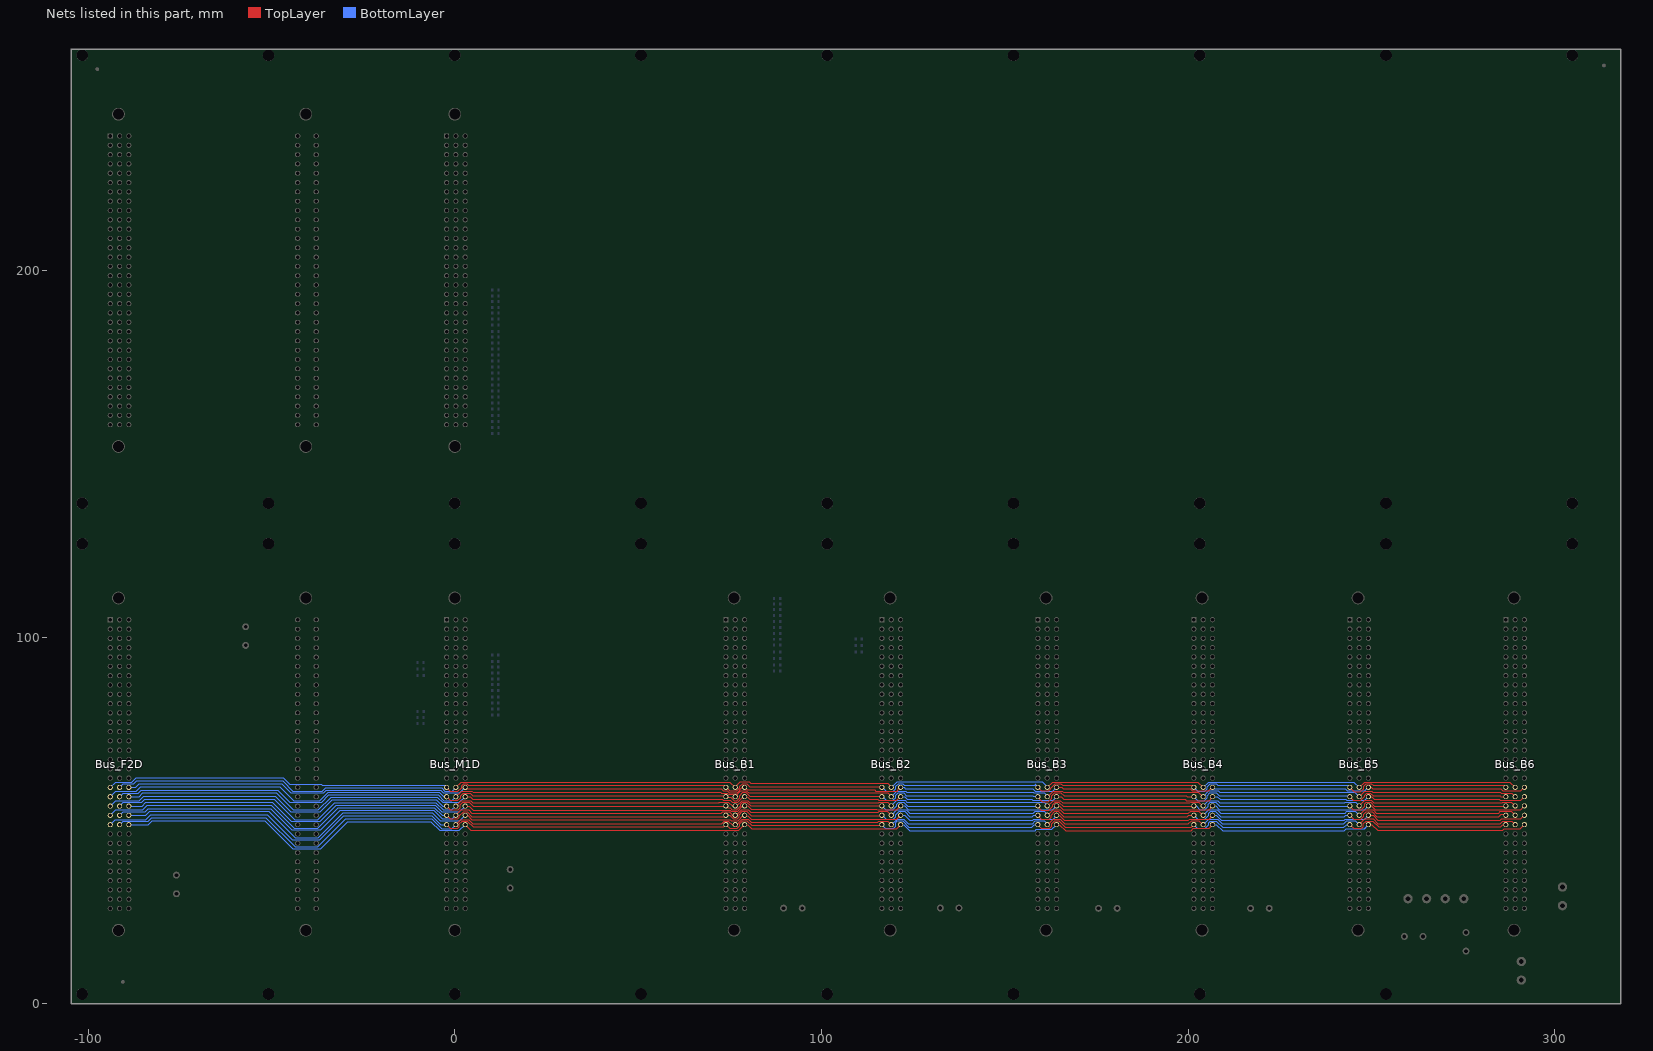
[diagram p0: the nets of this part, all layers, seen from the top]
# Altium PCB MISC67337.PcbDoc (part 3 of 7)
Units mm, origin at the board's own origin, x right, y up, seen from the top; angles counter-clockwise.
Board outline 422.71 x 260.35 mm, 4 copper layers (TopLayer, InternalPlane1, InternalPlane2, BottomLayer); 82 components, 143 nets, 1295 pads, 42 vias.

## Via types
v1: diameter 0.61, hole 0.305, TopLayer to BottomLayer, 42 vias

## Nets (pads, with @x,y where several pads share a name; then routed paths per layer and width w, separated by ;. In a path a pad name is that pad's centre, name@x,y a point inside that pad or via, vN(x,y) a via of type N, cw(c..) or ccw(c..) an arc to the next point about the centre after c; other vN are vias at no path point) (continued)
B_DSP1_XD0: Bus_B1.A19 Bus_B2.A19 Bus_B3.A19 Bus_B4.A19 Bus_B5.A19 Bus_B6.A19 Bus_F2D.A19 Bus_M1D.A19 | length 403.1
  TopLayer w0.254: Bus_M1D.A19@-2.24,58.974 -1.178,57.912 0.838,57.912 1.862,58.936 1.862,59.379 2.435,59.952 3.245,59.952 3.689,59.508 70.968,59.508 ; 72.996,59.508 70.968,59.508 ; Bus_B1.A19@73.955,58.993 73.44,59.508 70.968,59.508 ; Bus_B1.A19@73.96,59.12 75.065,58.015 76.9,58.015 77.785,58.9 77.785,59.248 78.508,59.971 79.704,59.971 80.457,59.217 Bus_B2.A19@116.505,59.217 ; Bus_B3.A19@159.05,58.993 160.004,58.039 161.036,58.039 161.06,58.015 161.995,58.015 162.568,58.588 162.568,58.814 163.774,60.02 165.329,60.02 165.849,59.499 168.021,59.499 ; 166.559,59.499 168.021,59.499 ; Bus_B4.A19@201.595,58.993 201.089,59.499 168.021,59.499 ; Bus_B5.A19@244.14,58.993 245.348,57.785 247.015,57.785 247.904,58.674 247.904,59.309 248.566,59.971 250.032,59.971 250.495,59.508 283.235,59.508 ; 283.945,59.508 283.235,59.508 ; Bus_B6.A19@286.685,58.993 286.17,59.508 283.235,59.508
  BottomLayer w0.254: Bus_F2D.A19@-93.97,58.974 -92.492,60.452 -88.138,60.452 -86.919,61.671 -46.838,61.671 -45.055,59.888 -36.47,59.888 -36.195,59.614 -2.88,59.614 Bus_M1D.A19@-2.24,58.974 ; Bus_B2.A19@116.632,59.055 117.713,57.974 119.634,57.974 120.269,58.609 120.269,59.244 121.058,60.033 122.162,60.033 122.631,59.564 155.981,59.564 ; 158.199,59.564 155.981,59.564 ; 158.199,60.033 Bus_B3.A19@159.177,59.055 ; Bus_B3.A19@159.05,58.993 158.479,59.564 155.981,59.564 ; Bus_B4.A19@201.595,58.993 202.676,57.912 204.597,57.912 205.232,58.547 205.232,59.182 206.021,59.971 207.635,59.971 208.102,59.504 242.519,59.504 ; 243.162,59.504 242.519,59.504 ; Bus_B5.A19@244.14,58.993 243.629,59.504 242.519,59.504
B_DSP1_XD1: Bus_B1.B19 Bus_B2.B19 Bus_B3.B19 Bus_B4.B19 Bus_B5.B19 Bus_B6.B19 Bus_F2D.B19 Bus_M1D.B19 | length 390.9
  TopLayer w0.254: Bus_M1D.B19@0.3,58.974 1.778,60.452 75.036,60.452 Bus_B1.B19@76.495,58.993 ; Bus_B1.B19@76.5,59.12 77.934,60.554 80.316,60.554 80.772,60.098 118.067,60.098 Bus_B2.B19@119.045,59.12 ; Bus_B3.B19@161.59,58.993 163.049,60.452 202.676,60.452 Bus_B4.B19@204.135,58.993 ; Bus_B5.B19@246.68,58.993 248.139,60.452 287.766,60.452 Bus_B6.B19@289.225,58.993
  BottomLayer w0.254: Bus_F2D.B19@-91.43,58.974 -90.452,59.952 -87.495,59.952 -86.69,60.757 -46.965,60.757 -44.204,57.996 -36.136,57.996 -35.23,58.903 -3.607,58.903 -2.7,57.996 -0.678,57.996 Bus_M1D.B19@0.3,58.974 ; Bus_B2.B19@119.172,59.055 120.631,60.514 160.258,60.514 Bus_B3.B19@161.717,59.055 ; Bus_B4.B19@204.135,58.993 205.594,60.452 245.221,60.452 Bus_B5.B19@246.68,58.993
B_DSP1_XD2: Bus_B1.C19 Bus_B2.C19 Bus_B3.C19 Bus_B4.C19 Bus_B5.C19 Bus_B6.C19 Bus_F2D.C19 Bus_M1D.C19 | length 392.7
  TopLayer w0.254: Bus_M1D.C19@2.84,58.564 72.627,58.564 73.176,58.015 74.351,58.015 74.835,57.531 76.991,57.531 Bus_B1.C19@78.453,58.993 ; Bus_B1.C19@79.035,58.993 79.167,58.993 79.823,58.337 114.554,58.337 ; 114.554,58.293 114.873,57.974 120.712,57.974 121.021,58.283 121.021,58.557 Bus_B2.C19@121.585,59.12 ; Bus_B3.C19@164.13,58.993 165.568,58.993 166.014,58.547 200.658,58.547 201.19,58.015 205.697,58.015 Bus_B4.C19@206.675,58.993 ; Bus_B5.C19@249.22,58.993 249.99,58.993 250.419,58.564 282.575,58.564 ; 283.653,58.564 282.575,58.564 ; 285.801,58.015 285.852,58.015 ; Bus_B6.C19@291.765,58.993 290.787,58.015 285.852,58.015 ; 282.575,58.564 285.303,58.564 285.852,58.015
  BottomLayer w0.254: Bus_F2D.C19@-88.89,58.974 -87.051,58.974 -86.055,59.969 -47.219,59.969 -44.78,57.531 -35.789,57.531 -35.077,58.242 -3.861,58.242 -3.15,57.531 1.397,57.531 Bus_M1D.C19@2.84,58.974 ; Bus_B2.C19@121.585,58.993 122.556,58.993 122.936,58.613 156.134,58.613 ; 157.226,58.613 156.134,58.613 ; Bus_B3.C19@164.257,59.055 163.114,57.912 158.369,57.912 157.668,58.613 156.134,58.613 ; Bus_B4.C19@206.675,58.993 207.113,58.555 240.259,58.555 ; 242.505,58.555 240.259,58.555 ; Bus_B5.C19@249.22,58.993 248.242,58.015 243.483,58.015 242.943,58.555 240.259,58.555
B_DSP1_XD3: Bus_B1.A20 Bus_B2.A20 Bus_B3.A20 Bus_B4.A20 Bus_B5.A20 Bus_B6.A20 Bus_F2D.A20 Bus_M1D.A20 | length 402.2
  TopLayer w0.254: Bus_M1D.A20@-2.24,56.434 -1.262,55.456 0.846,55.456 1.587,56.198 1.587,56.706 2.294,57.412 4.167,57.412 4.902,56.676 71.12,56.676 ; 72.63,56.676 71.12,56.676 ; Bus_B1.A20@73.955,56.453 73.732,56.676 71.12,56.676 ; Bus_B1.A20@73.96,56.453 74.152,56.261 75.209,56.261 76.173,55.297 76.913,55.297 77.724,56.109 77.724,56.769 78.564,57.609 79.402,57.609 80.435,56.575 113.538,56.575 ; 114.173,56.575 113.538,56.575 ; Bus_B2.A20@116.505,56.453 116.383,56.575 113.538,56.575 ; Bus_B3.A20@159.05,56.326 160.258,55.118 161.925,55.118 162.814,56.007 162.814,56.642 163.703,57.531 165.329,57.531 166.217,56.642 198.476,56.642 ; 198.957,56.642 198.476,56.642 ; Bus_B4.A20@201.595,56.326 201.533,56.388 Bus_B4.A20@201.53,56.388 ; Bus_B4.A20@201.595,56.453 Bus_B4.A20@201.53,56.388 ; Bus_B5.A20@244.14,56.453 245.118,55.475 247.118,55.475 248.158,56.515 248.158,56.896 248.693,57.431 249.706,57.431 250.461,56.676 282.677,56.676 ; 283.31,56.676 282.677,56.676 ; Bus_B6.A20@286.685,56.453 285.344,56.453 285.12,56.676 282.677,56.676 ; 198.476,56.642 199.517,56.642 199.771,56.388 Bus_B4.A20@201.53,56.388
  BottomLayer w0.254: Bus_F2D.A20@-93.97,56.434 -92.492,57.912 -86.919,57.912 -85.649,59.182 -47.727,59.182 -43.917,55.372 -36.805,55.372 -34.544,57.633 -4.242,57.633 -3.043,56.434 Bus_M1D.A20@-2.24,56.434 ; Bus_B2.A20@116.632,56.515 117.713,55.434 119.507,55.434 120.269,56.196 120.269,56.831 120.944,57.506 122.403,57.506 123.196,56.713 155.296,56.713 ; 156.464,56.713 155.296,56.713 ; Bus_B3.A20@159.05,56.453 Bus_B3.A20@158.988,56.515 ; Bus_B3.A20@159.177,56.515 Bus_B3.A20@158.988,56.515 ; Bus_B4.A20@201.595,56.453 202.676,55.372 204.47,55.372 205.232,56.134 205.232,56.769 205.994,57.531 207.696,57.531 208.568,56.659 241.3,56.659 ; 241.427,56.659 241.3,56.659 ; Bus_B5.A20@244.14,56.453 243.934,56.659 241.3,56.659 ; 155.296,56.713 157.598,56.713 157.796,56.515 Bus_B3.A20@158.988,56.515
B_DSP1_XD4: Bus_B1.B20 Bus_B2.B20 Bus_B3.B20 Bus_B4.B20 Bus_B5.B20 Bus_B6.B20 Bus_F2D.B20 Bus_M1D.B20 | length 395
  TopLayer w0.254: Bus_M1D.B20@0.3,56.434 1.862,57.996 4.653,57.996 5.029,57.62 72.531,57.62 72.72,57.431 74.36,57.431 74.667,57.125 75.824,57.125 Bus_B1.B20@76.495,56.453 ; Bus_B1.B20@76.5,56.453 78.062,58.015 79.57,58.015 79.689,57.896 ; 79.85,57.736 79.689,57.896 ; 114.349,57.456 113.716,57.456 ; Bus_B2.B20@119.045,56.453 118.042,57.456 113.716,57.456 ; Bus_B3.B20@161.59,56.326 163.201,57.937 165.748,57.937 166.091,57.595 202.852,57.595 ; 202.852,57.609 Bus_B4.B20@204.135,56.326 ; Bus_B5.B20@246.68,56.453 248.139,57.912 250.101,57.912 250.393,57.62 285.18,57.62 285.369,57.431 288.247,57.431 Bus_B6.B20@289.225,56.453 ; 79.689,57.896 80.129,57.456 113.716,57.456
  BottomLayer w0.254: Bus_F2D.B20@-91.43,56.434 -90.452,57.412 -86.301,57.412 -85.446,58.268 -48.311,58.268 -45.009,54.966 -36.297,54.966 -34.315,56.947 -4.521,56.947 -2.946,55.372 -0.762,55.372 Bus_M1D.B20@0.3,56.434 ; Bus_B2.B20@119.172,56.515 120.569,57.912 122.966,57.912 123.215,57.663 155.448,57.663 ; 156.972,57.663 155.448,57.663 ; Bus_B3.B20@161.717,56.515 160.726,57.506 157.948,57.506 157.791,57.663 155.448,57.663 ; Bus_B4.B20@204.135,56.453 205.697,58.015 208.278,58.015 208.686,57.607 241.605,57.607 ; 241.935,57.607 241.605,57.607 ; Bus_B5.B20@246.68,56.453 245.526,57.607 241.605,57.607
B_DSP1_XD5: Bus_B1.C20 Bus_B2.C20 Bus_B3.C20 Bus_B4.C20 Bus_B5.C20 Bus_B6.C20 Bus_F2D.C20 Bus_M1D.C20 | length 393.8
  TopLayer w0.254: Bus_M1D.C20@2.84,56.434 4.201,56.434 4.902,55.732 72.009,55.732 ; 72.217,55.732 72.009,55.732 ; 113.473,55.695 113.005,55.695 ; Bus_B2.C20@121.585,56.453 120.58,55.448 115.646,55.448 115.4,55.695 113.005,55.695 ; Bus_B3.C20@164.13,56.453 165.391,56.453 166.154,55.69 198.222,55.69 ; 198.563,55.69 198.222,55.69 ; Bus_B4.C20@206.675,56.326 205.746,55.397 199.492,55.397 199.199,55.69 198.222,55.69 ; Bus_B5.C20@249.22,56.453 250.1,56.453 250.82,55.732 282.677,55.732 ; 282.891,55.732 282.677,55.732 ; Bus_B6.C20@291.765,56.453 290.787,55.475 285.166,55.475 284.909,55.732 282.677,55.732 ; 72.009,55.732 72.919,55.732 73.177,55.474 75.133,55.474 75.716,54.891 77.192,54.891 78.754,56.453 79.742,56.453 80.5,55.695 113.005,55.695
  BottomLayer w0.254: Bus_F2D.C20@-88.89,56.434 -86.085,56.434 -85.039,57.48 -48.692,57.48 -44.044,52.832 -37.211,52.832 -33.731,56.312 -4.775,56.312 -3.335,54.872 1.278,54.872 Bus_M1D.C20@2.84,56.434 ; Bus_B2.C20@121.585,56.453 122.744,56.453 123.435,55.762 124.358,55.762 ; 123.571,55.762 124.358,55.762 ; 155.956,55.762 155.397,55.762 ; Bus_B3.C20@164.257,56.515 163.216,55.474 157.694,55.474 157.406,55.762 155.397,55.762 ; Bus_B4.C20@206.675,56.453 208.037,56.453 208.78,55.71 243.071,55.71 243.307,55.475 248.242,55.475 Bus_B5.C20@249.22,56.453 ; 124.358,55.762 155.397,55.762
B_DSP1_XD6: Bus_B1.A21 Bus_B2.A21 Bus_B3.A21 Bus_B4.A21 Bus_B5.A21 Bus_B6.A21 Bus_F2D.A21 Bus_M1D.A21 | length 398.5
  TopLayer w0.254: Bus_M1D.A21@-2.24,53.894 -1.262,52.916 0.973,52.916 1.524,53.467 1.524,54.229 2.167,54.872 3.98,54.872 5.007,53.844 Bus_B1.A21@73.309,53.844 ; Bus_B1.A21@73.96,53.913 74.457,53.416 75.133,53.416 75.614,52.935 76.9,52.935 77.978,54.013 77.978,54.361 78.583,54.966 79.654,54.966 80.687,53.933 116.485,53.933 Bus_B2.A21@116.505,53.913 ; Bus_B3.A21@159.05,53.786 160.028,52.808 162.028,52.808 163.068,53.848 163.068,54.234 163.825,54.991 164.77,54.991 165.976,53.785 201.467,53.785 Bus_B4.A21@201.595,53.913 ; Bus_B5.A21@244.14,53.913 245.118,52.935 247.245,52.935 248.158,53.848 248.158,54.483 248.566,54.891 249.782,54.891 250.829,53.844 282.194,53.844 ; 282.421,53.844 282.194,53.844 ; Bus_B6.A21@286.685,53.913 286.616,53.844 282.194,53.844
  BottomLayer w0.254: Bus_F2D.A21@-93.97,53.894 -92.492,55.372 -86.03,55.372 -84.861,56.54 -48.997,56.54 -44.78,52.324 -36.703,52.324 -33.452,55.575 -5.004,55.575 -3.323,53.894 Bus_M1D.A21@-2.24,53.894 ; Bus_B2.A21@116.632,53.975 116.632,53.802 117.602,52.832 119.412,52.832 120.523,53.943 120.523,54.418 121.058,54.953 122.441,54.953 123.532,53.861 155.067,53.861 ; 155.932,53.861 155.067,53.861 ; Bus_B3.A21@159.05,53.913 158.998,53.861 155.067,53.861 ; Bus_B4.A21@201.595,53.913 202.179,53.913 203.157,52.935 204.54,52.935 205.486,53.881 205.486,54.356 206.045,54.915 207.594,54.915 208.695,53.814 240.538,53.814 ; 240.895,53.814 240.538,53.814 ; Bus_B5.A21@244.14,53.913 244.041,53.814 240.538,53.814
B_DSP1_XD7: Bus_B1.B21 Bus_B2.B21 Bus_B3.B21 Bus_B4.B21 Bus_B5.B21 Bus_B6.B21 Bus_F2D.B21 Bus_M1D.B21 | length 396.8
  TopLayer w0.254: Bus_M1D.B21@0.3,53.894 1.778,55.372 4.319,55.372 4.902,54.788 72.085,54.788 72.188,54.891 74.649,54.891 75.627,53.913 76.9,53.913 78.359,55.372 79.934,55.372 80.492,54.814 113.233,54.814 ; 113.665,54.814 113.233,54.814 ; Bus_B2.B21@119.045,53.913 118.043,54.915 115.748,54.915 115.647,54.814 113.233,54.814 ; Bus_B3.B21@161.59,53.786 163.201,55.397 165.151,55.397 165.811,54.737 198.323,54.737 ; 198.603,54.737 198.323,54.737 ; Bus_B4.B21@204.135,53.786 202.93,54.991 200.711,54.991 200.457,54.737 198.323,54.737 ; Bus_B5.B21@246.68,53.913 248.242,55.475 249.985,55.475 250.672,54.788 282.575,54.788 ; 282.98,54.788 282.575,54.788 ; 285.826,54.991 285.852,54.991 ; Bus_B6.B21@289.225,53.913 288.147,54.991 285.852,54.991 ; 282.575,54.788 285.649,54.788 285.852,54.991
  BottomLayer w0.254: Bus_F2D.B21@-91.43,53.894 -90.358,54.966 -85.42,54.966 -84.607,55.778 -49.276,55.778 -43.663,50.165 -37.338,50.165 -32.664,54.839 -5.131,54.839 -3.124,52.832 -0.762,52.832 Bus_M1D.B21@0.3,53.894 ; Bus_B2.B21@119.045,53.913 120.555,55.423 122.834,55.423 123.304,54.953 160.739,54.953 Bus_B3.B21@161.717,53.975 ; Bus_B4.B21@204.135,53.913 205.569,55.347 208.051,55.347 208.636,54.762 241.122,54.762 ; 241.581,54.762 241.122,54.762 ; Bus_B5.B21@246.68,53.913 245.702,54.891 242.875,54.891 242.746,54.762 241.122,54.762
B_DSP1_XD8: Bus_B1.C21 Bus_B2.C21 Bus_B3.C21 Bus_B4.C21 Bus_B5.C21 Bus_B6.C21 Bus_F2D.C21 Bus_M1D.C21 | length 395.3
  TopLayer w0.254: Bus_M1D.C21@2.84,53.894 3.916,53.894 5.053,52.757 75.081,52.757 75.309,52.529 77.141,52.529 78.526,53.913 Bus_B1.C21@79.035,53.913 79.945,53.913 80.805,53.053 115.121,53.053 115.316,52.857 120.529,52.857 Bus_B2.C21@121.585,53.913 ; Bus_B3.C21@164.13,53.913 164.857,53.913 165.938,52.832 199.975,52.832 200,52.857 205.746,52.857 Bus_B4.C21@206.675,53.786 ; Bus_B5.C21@249.22,53.913 250.023,53.913 251.036,52.901 281.889,52.901 ; 282.129,52.901 281.889,52.901 ; Bus_B6.C21@291.765,53.913 290.753,52.901 281.889,52.901
  BottomLayer w0.254: Bus_F2D.C21@-88.89,53.894 -85.247,53.894 -84.226,54.915 -49.759,54.915 -44.602,49.759 -36.627,49.759 -32.258,54.127 -5.309,54.127 -3.513,52.332 1.278,52.332 Bus_M1D.C21@2.84,53.894 ; Bus_B2.C21@121.585,53.913 122.744,53.913 123.746,52.911 152.552,52.911 ; 155.764,52.911 152.552,52.911 ; Bus_B3.C21@164.13,53.913 163.128,52.911 152.552,52.911 ; Bus_B3.C21@164.163,53.881 Bus_B3.C21@164.257,53.975 ; Bus_B4.C21@206.675,53.913 207.605,53.913 208.583,52.935 248.242,52.935 Bus_B5.C21@249.22,53.913
B_DSP1_XD9: Bus_B1.A22 Bus_B2.A22 Bus_B3.A22 Bus_B4.A22 Bus_B5.A22 Bus_B6.A22 Bus_F2D.A22 Bus_M1D.A22 | length 405.9
  TopLayer w0.254: Bus_M1D.A22@-2.24,51.354 -1.262,50.376 0.846,50.376 1.278,50.808 1.278,51.189 2.421,52.332 3.37,52.332 4.69,51.013 70.51,51.013 ; 72.001,51.013 70.51,51.013 ; 112.166,51.292 112.039,51.292 ; Bus_B2.A22@116.505,51.373 116.424,51.292 112.039,51.292 ; Bus_B3.A22@159.05,51.246 160.028,50.268 162.155,50.268 162.687,50.8 162.687,51.435 163.703,52.451 164.541,52.451 166.065,50.927 199.808,50.927 200.254,51.373 Bus_B4.A22@201.595,51.373 ; Bus_B5.A22@244.14,51.373 245.221,50.292 247.142,50.292 247.904,51.054 247.904,51.689 248.566,52.351 250.188,52.351 251.527,51.013 280.416,51.013 ; 281.432,51.013 280.416,51.013 ; Bus_B6.A22@286.685,51.373 286.369,51.689 285.42,51.689 284.743,51.013 280.416,51.013 ; 70.51,51.013 73.595,51.013 Bus_B1.A22@73.955,51.373 74.968,51.373 75.946,50.395 76.989,50.395 77.597,51.003 77.597,51.562 78.461,52.426 79.68,52.426 80.814,51.292 112.039,51.292
  BottomLayer w0.254: Bus_F2D.A22@-93.97,51.354 -92.492,52.832 -85.141,52.832 -83.896,54.077 -50.038,54.077 -43.84,47.879 -37.313,47.879 -31.725,53.467 -5.563,53.467 -3.45,51.354 Bus_M1D.A22@-2.24,51.354 ; Bus_B2.A22@116.632,51.435 117.713,50.354 119.634,50.354 120.269,50.989 120.269,51.497 121.198,52.426 122.682,52.426 124.097,51.01 153.441,51.01 ; 154.305,51.01 153.441,51.01 ; Bus_B3.A22@159.05,51.373 Bus_B3.A22@158.988,51.435 ; Bus_B3.A22@159.177,51.435 Bus_B3.A22@158.988,51.435 ; Bus_B4.A22@201.595,51.373 202.676,50.292 204.597,50.292 205.697,51.392 205.697,51.9 206.248,52.451 207.493,52.451 208.975,50.968 238.658,50.968 ; 239.268,50.968 238.658,50.968 ; Bus_B5.A22@244.14,51.373 243.002,51.373 242.597,50.968 238.658,50.968 ; 153.441,51.01 157.487,51.01 157.912,51.435 Bus_B3.A22@158.988,51.435
B_DSP1_XD10: Bus_B1.B22 Bus_B2.B22 Bus_B3.B22 Bus_B4.B22 Bus_B5.B22 Bus_B6.B22 Bus_F2D.B22 Bus_M1D.B22 | length 401.4
  TopLayer w0.254: Bus_M1D.B22@0.3,51.354 1.778,52.832 3.798,52.832 4.674,51.957 ; 4.648,51.957 4.674,51.957 ; 112.903,52.172 111.912,52.172 ; Bus_B2.B22@119.045,51.373 117.967,52.451 115.748,52.451 115.469,52.172 111.912,52.172 ; Bus_B3.B22@161.59,51.246 163.201,52.857 165.1,52.857 166.078,51.88 197.587,51.88 ; 197.841,51.88 197.587,51.88 ; Bus_B4.B22@204.135,51.246 202.93,52.451 200.685,52.451 200.114,51.88 197.587,51.88 ; Bus_B5.B22@246.68,51.373 248.139,52.832 250.495,52.832 251.37,51.957 281.457,51.957 ; 281.813,51.957 281.457,51.957 ; Bus_B6.B22@289.225,51.373 288.147,52.451 285.217,52.451 284.722,51.957 281.457,51.957 ; 4.674,51.957 72.644,51.957 73.038,52.351 74.801,52.351 76.251,50.902 78.257,52.908 80.01,52.908 80.746,52.172 111.912,52.172
  BottomLayer w0.254: Bus_F2D.B22@-91.43,51.354 -90.452,52.332 -84.396,52.332 -83.566,53.162 -50.19,53.162 -44.399,47.371 -36.601,47.371 -31.293,52.68 -5.74,52.68 -3.437,50.376 -0.678,50.376 Bus_M1D.B22@0.3,51.354 ; Bus_B2.B22@119.172,51.435 120.569,52.832 123.176,52.832 124.047,51.961 153.492,51.961 ; 155.194,51.961 153.492,51.961 ; Bus_B3.B22@161.717,51.435 160.726,52.426 158.267,52.426 157.803,51.961 153.492,51.961 ; Bus_B4.B22@204.135,51.373 205.657,52.896 207.963,52.896 208.941,51.917 239.522,51.917 ; 240.157,51.917 239.522,51.917 ; Bus_B5.B22@246.68,51.373 245.602,52.451 243.357,52.451 242.823,51.917 239.522,51.917
B_DSP1_XD11: Bus_B1.C22 Bus_B2.C22 Bus_B3.C22 Bus_B4.C22 Bus_B5.C22 Bus_B6.C22 Bus_F2D.C22 Bus_M1D.C22 | length 397
  TopLayer w0.254: Bus_M1D.C22@2.84,51.354 3.492,51.354 4.631,50.216 73.176,50.216 73.177,50.217 75.132,50.217 75.438,49.911 77.267,49.911 78.729,51.373 Bus_B1.C22@79.035,51.373 ; Bus_B1.C22@79.035,50.885 79.458,51.308 79.883,51.308 80.848,50.343 120.555,50.343 Bus_B2.C22@121.585,51.373 ; Bus_B3.C22@164.13,51.373 164.857,51.373 166.255,49.975 196.647,49.975 ; 197.039,49.975 196.647,49.975 ; Bus_B4.C22@206.675,51.246 205.746,50.317 200.431,50.317 200.089,49.975 196.647,49.975 ; Bus_B5.C22@249.22,51.373 250.455,51.373 251.759,50.069 285.197,50.069 285.523,50.395 290.787,50.395 Bus_B6.C22@291.765,51.373
  BottomLayer w0.254: Bus_F2D.C22@-88.89,51.354 -84.282,51.354 -83.21,52.426 -50.724,52.426 -43.51,45.212 -37.211,45.212 -30.404,52.019 -6.096,52.019 -3.988,49.911 1.397,49.911 Bus_M1D.C22@2.84,51.354 ; Bus_B2.C22@121.585,51.373 122.795,51.373 124.108,50.06 152.476,50.06 ; 153.924,50.06 152.476,50.06 ; Bus_B3.C22@164.257,51.435 163.176,50.354 157.988,50.354 157.694,50.06 152.476,50.06 ; Bus_B4.C22@206.675,51.373 207.758,51.373 209.111,50.02 242.603,50.02 242.875,50.292 248.139,50.292 Bus_B5.C22@249.22,51.373
B_DSP1_XD12: Bus_B1.A23 Bus_B2.A23 Bus_B3.A23 Bus_B4.A23 Bus_B5.A23 Bus_B6.A23 Bus_F2D.A23 Bus_M1D.A23 | length 408.9
  TopLayer w0.254: Bus_M1D.A23@-2.24,48.814 -1.262,47.836 0.84,47.836 1.278,48.274 1.278,49.03 2.04,49.792 3.396,49.792 5.007,48.181 6.833,48.181 ; 5.396,48.181 6.833,48.181 ; Bus_B1.A23@73.955,48.718 73.841,48.718 73.303,48.181 6.833,48.181 ; Bus_B1.A23@73.96,48.833 74.938,47.855 77.065,47.855 77.724,48.514 77.724,49.022 78.588,49.886 79.705,49.886 80.941,48.65 109.703,48.65 ; 111.531,48.65 109.703,48.65 ; Bus_B2.A23@116.505,48.833 116.322,48.65 109.703,48.65 ; Bus_B3.A23@159.05,48.706 159.901,47.855 162.282,47.855 162.814,48.387 162.814,49.022 163.703,49.911 164.719,49.911 166.56,48.07 196.19,48.07 ; 196.469,48.07 196.19,48.07 ; Bus_B4.A23@201.595,48.706 Bus_B4.A23@201.468,48.706 ; Bus_B4.A23@201.595,48.833 Bus_B4.A23@201.468,48.706 ; Bus_B5.A23@244.14,48.833 245.196,47.777 247.294,47.777 247.777,48.26 247.777,49.022 248.566,49.811 250.341,49.811 251.971,48.181 252.476,48.181 ; 252.184,48.181 252.476,48.181 ; 280.162,48.181 279.908,48.181 ; Bus_B6.A23@286.685,48.833 285.891,48.833 285.239,48.181 279.908,48.181 ; 196.19,48.07 200.832,48.07 Bus_B4.A23@201.468,48.706 ; 252.476,48.181 279.908,48.181
  BottomLayer w0.254: Bus_F2D.A23@-93.97,48.814 -92.585,50.198 -84.295,50.198 -82.931,51.562 -51.13,51.562 -44.272,44.704 -36.779,44.704 -30.226,51.257 -6.248,51.257 -3.805,48.814 Bus_M1D.A23@-2.24,48.814 ; Bus_B2.A23@116.505,48.833 117.483,47.855 119.675,47.855 120.269,48.449 120.269,49.403 120.701,49.835 122.149,49.835 123.824,48.159 152.73,48.159 ; 153.389,48.159 152.73,48.159 ; Bus_B3.A23@159.05,48.833 158.104,48.833 157.43,48.159 152.73,48.159 ; Bus_B3.A23@159.05,48.895 Bus_B3.A23@159.177,48.895 ; Bus_B4.A23@201.595,48.833 202.573,47.855 204.7,47.855 205.613,48.768 205.613,49.403 206.021,49.811 207.745,49.811 209.433,48.123 238.125,48.123 ; 238.352,48.123 238.125,48.123 ; Bus_B5.A23@244.14,48.833 243.245,48.833 242.535,48.123 238.125,48.123
B_DSP1_XD13: Bus_B1.B23 Bus_B2.B23 Bus_B3.B23 Bus_B4.B23 Bus_B5.B23 Bus_B6.B23 Bus_F2D.B23 Bus_M1D.B23 | length 404.9
  TopLayer w0.254: Bus_M1D.B23@0.3,48.814 1.684,50.198 3.777,50.198 4.85,49.125 72.772,49.125 73.458,49.811 74.649,49.811 75.627,48.833 Bus_B1.B23@76.495,48.833 ; Bus_B1.B23@76.5,48.833 76.849,48.833 78.359,50.343 80.061,50.343 80.873,49.53 110.795,49.53 ; 112.141,49.53 110.795,49.53 ; Bus_B2.B23@119.045,48.833 118.067,49.811 115.673,49.811 115.392,49.53 110.795,49.53 ; Bus_B3.B23@161.59,48.706 163.201,50.317 165.1,50.317 166.395,49.023 196.545,49.023 ; 197.079,49.023 196.545,49.023 ; Bus_B4.B23@204.135,48.706 202.93,49.911 200.965,49.911 200.076,49.023 196.545,49.023 ; Bus_B5.B23@246.68,48.833 248.242,50.395 250.493,50.395 251.764,49.125 279.857,49.125 ; 280.67,49.125 279.857,49.125 ; Bus_B6.B23@289.225,48.833 288.274,49.784 288.138,49.784 288.111,49.811 285.802,49.811 285.116,49.125 279.857,49.125
  BottomLayer w0.254: Bus_F2D.B23@-91.43,48.814 -90.452,49.792 -83.583,49.792 -82.677,50.698 -51.486,50.698 -43.523,42.736 -37.351,42.736 -29.667,50.419 -6.299,50.419 -3.539,47.658 -2.821,47.658 ; -2.829,47.65 -2.821,47.658 ; Bus_M1D.B23@0.3,48.814 -0.856,47.658 -2.821,47.658 ; Bus_B2.B23@119.045,48.833 119.11,48.833 120.631,50.354 122.442,50.354 123.686,49.11 152.248,49.11 ; 153.924,49.11 152.248,49.11 ; Bus_B3.B23@161.717,48.895 160.739,49.873 158.356,49.873 157.593,49.11 152.248,49.11 ; Bus_B4.B23@204.135,48.833 205.594,50.292 208.051,50.292 209.272,49.072 242.518,49.072 243.281,49.835 245.678,49.835 Bus_B5.B23@246.68,48.833
B_DSP1_XD14: Bus_B1.C23 Bus_B2.C23 Bus_B3.C23 Bus_B4.C23 Bus_B5.C23 Bus_B6.C23 Bus_F2D.C23 Bus_M1D.C23 | length 400.2
  TopLayer w0.254: 3.799,47.855 Bus_M1D.C23@2.84,48.814 4.383,47.271 77.473,47.271 Bus_B1.C23@78.843,48.641 ; Bus_B1.C23@79.035,48.833 79.97,48.833 81.034,47.769 120.504,47.769 ; 120.504,47.752 Bus_B2.C23@121.585,48.833 ; Bus_B3.C23@164.13,48.833 164.908,48.833 166.623,47.118 196.037,47.118 ; 196.658,47.118 196.037,47.118 ; 201.422,47.777 201.473,47.777 ; Bus_B4.C23@206.675,48.706 205.746,47.777 201.473,47.777 ; Bus_B5.C23@249.22,48.833 250.15,48.833 251.746,47.237 255.448,47.237 ; 255.245,47.237 255.448,47.237 ; Bus_B6.C23@291.765,48.833 290.582,47.65 286.283,47.65 285.87,47.237 255.448,47.237 ; 196.037,47.118 200.813,47.118 201.473,47.777
  BottomLayer w0.254: Bus_F2D.C23@-88.89,48.814 -83.545,48.814 -82.499,49.86 -51.816,49.86 -44.247,42.291 -36.5,42.291 -29.134,49.657 -6.553,49.657 -4.14,47.244 -2.653,47.244 -2.645,47.252 1.278,47.252 Bus_M1D.C23@2.84,48.814 ; Bus_B2.C23@121.585,48.833 122.414,48.833 124.038,47.209 152.705,47.209 ; 152.97,47.209 152.705,47.209 ; Bus_B3.C23@164.13,48.833 162.846,47.549 158.648,47.549 158.309,47.209 152.705,47.209 ; Bus_B3.C23@164.163,48.801 Bus_B3.C23@164.257,48.895 ; Bus_B4.C23@206.675,48.833 207.758,48.833 209.416,47.175 242.628,47.175 243.205,47.752 248.139,47.752 Bus_B5.C23@249.22,48.833 248.242,47.855